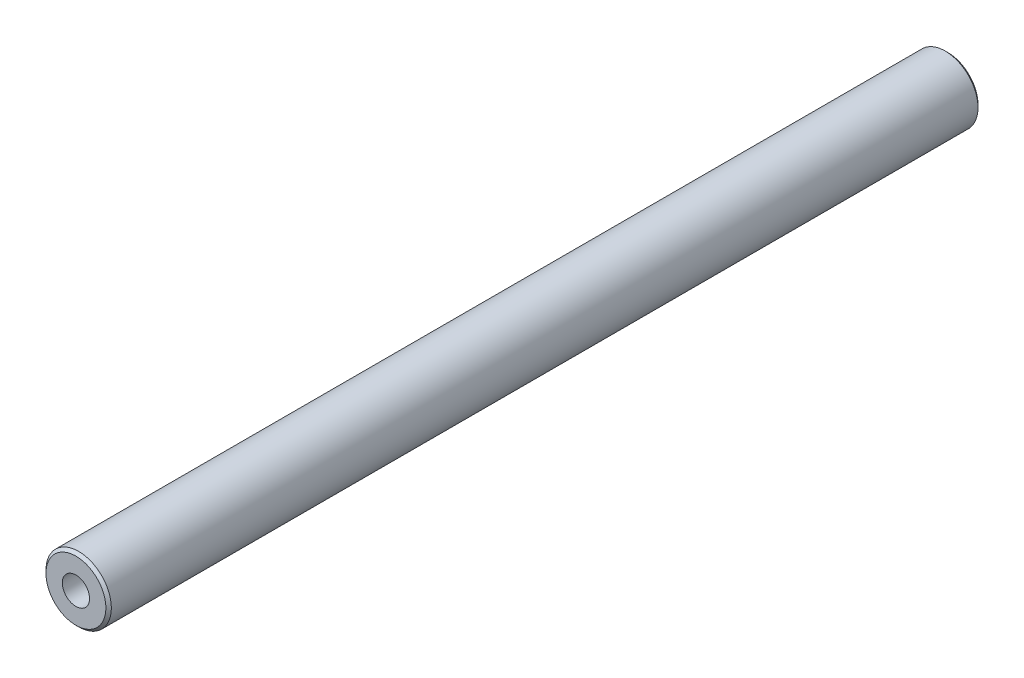
from build123d import *

# Parameters (mm, degrees)
SKETCH1_R             = 6
BOSS_EXTRUDE1_DEPTH   = 160
M6_TAPPED_HOLE1_D     = 5
M6_TAPPED_HOLE1_DEPTH = 15
M6_TAPPED_HOLE1_TIP   = 1.502151548
CHAMFER1_SIZE         = 0.5


with BuildPart() as part:
    # Sketch1 → Boss-Extrude1 (new body)
    with BuildSketch(Plane.XY):
        Circle(SKETCH1_R)
    extrude(amount=BOSS_EXTRUDE1_DEPTH)

    # M6 Tapped Hole1
    with Locations(Plane.XY.offset(160)):
        with Locations((0, 0)):
            Hole(M6_TAPPED_HOLE1_D / 2, depth=M6_TAPPED_HOLE1_DEPTH)
            with Locations((0, 0, -(M6_TAPPED_HOLE1_DEPTH + M6_TAPPED_HOLE1_TIP / 2))):  # 118° drill point
                Cone(0, M6_TAPPED_HOLE1_D / 2, M6_TAPPED_HOLE1_TIP, mode=Mode.SUBTRACT)

    # Chamfer1
    chamfer1_edges = [part.edges().sort_by_distance(p)[0] for p in [
        (-6, 0, 0),
        (-6, 0, 160),
    ]]
    chamfer(chamfer1_edges, length=CHAMFER1_SIZE)


solid = part.part
